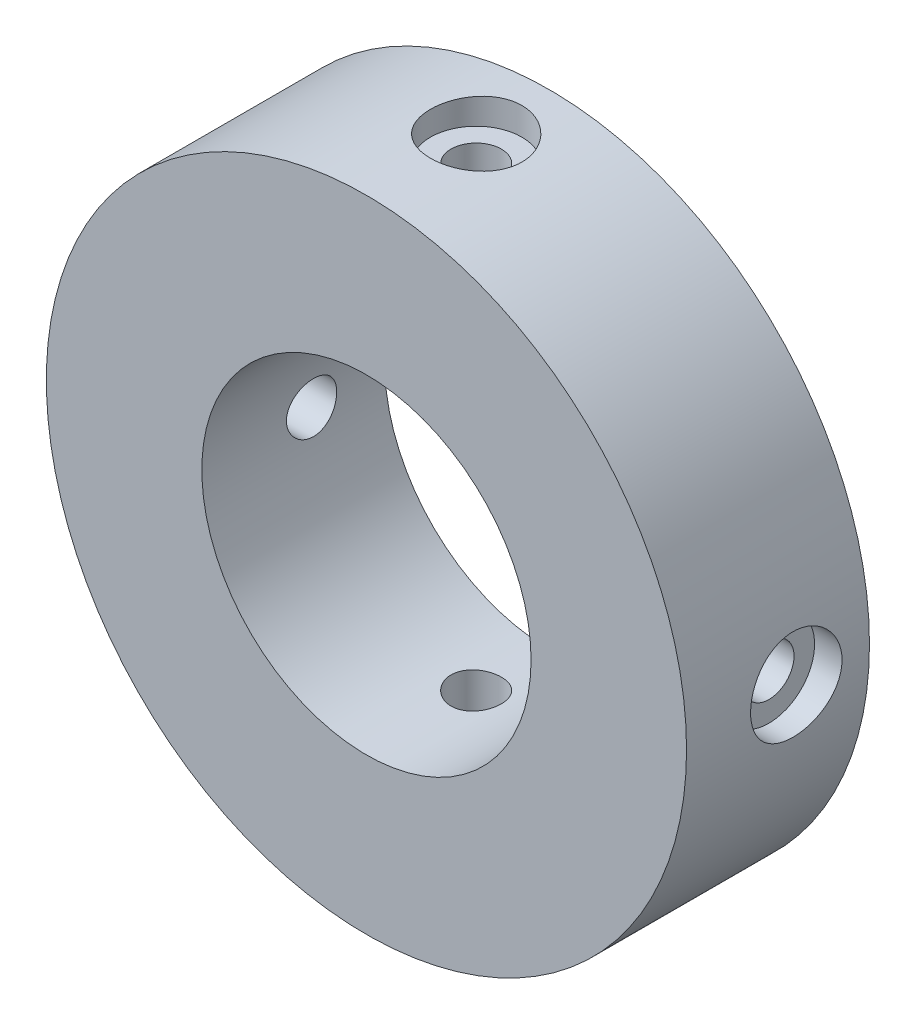
SolidWorks part; units mm, degrees
ref_plane "前视基准面" through (0, 0, 0) normal (0, 0, 1) x (1, 0, 0)
ref_plane "上视基准面" through (0, 0, 0) normal (0, 1, 0) x (1, 0, 0)
ref_plane "右视基准面" through (0, 0, 0) normal (1, 0, 0) x (0, 0, -1)
sketch "草图1" plane through (0, 0, 0) normal (0, 0, 1) x (1, 0, 0)
  circle A0 centre (0, 0) radius 35
  circle A1 centre (0, 0) radius 18
  dimension "D1" = 70
  dimension "D2" = 36
extrude "凸台-拉伸1" add sketch "草图1" along normal blind 20
sketch "草图5" plane through (0, 0, 0) normal (0, 1, 0) x (1, 0, 0)
  line L0 (0, 0) -> (0, -8) construction
  line L1 (35, 0) -> (-35, 0) construction
  circle A0 centre (0, -8) radius 2.75
  dimension "D1" = 5.5
  dimension "D2" = 8
extrude "切除-拉伸1" cut sketch "草图5" against normal blind 33
sketch "草图6" plane through (0, 0, 0) normal (0, 1, 0) x (1, 0, 0)
  circle A0 centre (0, -8) radius 5
  dimension "D1" = 10
extrude "切除-拉伸3" cut sketch "草图6" against normal blind 33 from offset 32 offset against normal yes
pattern_circular "阵列(圆周)1" count 4 over 360 about axis through (0, 0, 0) along (0, 0, 1) of "切除-拉伸1", "切除-拉伸3"
sketch "草图3" plane through (0, 0, 0) normal (0, 0, 1) x (1, 0, 0)
  line L0 (0, 0) -> (21.2132, 21.2132) construction
  line L1 (0, 0) -> (12.7817, 0) construction
  dimension "D1" = 30
  dimension "D2" = 45
hole_wizard "M4x0.7 螺纹孔1" positions "3D草图1" profile "草图7" tap size "M4x0.7" standard "BSI"
sketch3d "3D草图1"
  point P0 (21.2132, 21.2132, 0)
sketch "草图7" plane through (21.2132, 21.2132, 0) normal (1, 0, 0) x (0, 1, 0)
  line L0 (0, 0) -> (0, 11.0914)
  line L1 (0, 11.0914) -> (1.65, 10.1)
  line L2 (1.65, 10.1) -> (1.65, 0)
  line L5 (1.65, 0) -> (0, 0)
  line L10 (0, 11.0914) -> (-1.65, 10.1) construction
  line L11 (0, -6.35) -> (0, 107.95) construction
  dimension "螺纹孔钻头直径" = 3.3
  dimension "螺纹孔钻头深度" = 10.1
  dimension "导头角度" = 118
cosmetic thread "孔螺蚊线1" parameters "D1"=8, "D2"=4
pattern_circular "阵列(圆周)2" count 4 over 360 about axis through (0, 0, 0) along (0, 0, 1) of "M4x0.7 螺纹孔1"
cosmetic thread "孔螺蚊线2" parameters "D1"=8, "D2"=4
cosmetic thread "孔螺蚊线3" parameters "D1"=8, "D2"=4
cosmetic thread "孔螺蚊线4" parameters "D1"=8, "D2"=4
